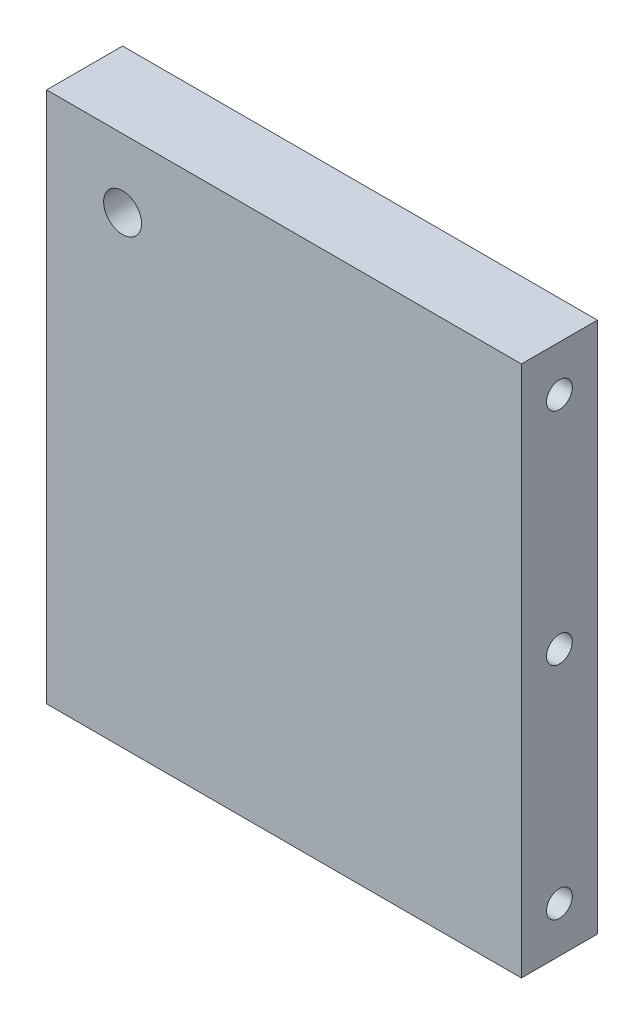
from build123d import *

# Parameters (mm, degrees)
SKETCH1_W              = 125
SKETCH1_H              = 140
BOSS_EXTRUDE1_DEPTH    = 20
M10_TAPPED_HOLE1_D     = 8.5
M10_TAPPED_HOLE1_DEPTH = 35
M10_TAPPED_HOLE1_TIP   = 2.553657631
M8_TAPPED_HOLE1_D      = 6.8
M8_TAPPED_HOLE1_DEPTH  = 22.25
M8_TAPPED_HOLE1_TIP    = 2.042926105
SKETCH6_R              = 5
CUT_EXTRUDE1_DEPTH     = 96.949205312


with BuildPart() as part:
    # Sketch1 → Boss-Extrude1 (new body)
    with BuildSketch(Plane.XY):
        Rectangle(SKETCH1_W, SKETCH1_H)
    extrude(amount=BOSS_EXTRUDE1_DEPTH)

    # M10 Tapped Hole1
    with Locations(Plane.ZY.offset(62.5)):
        with Locations((10, 40), (10, 0), (10, -40)):
            Hole(M10_TAPPED_HOLE1_D / 2, depth=M10_TAPPED_HOLE1_DEPTH)
            with Locations((0, 0, -(M10_TAPPED_HOLE1_DEPTH + M10_TAPPED_HOLE1_TIP / 2))):  # 118° drill point
                Cone(0, M10_TAPPED_HOLE1_D / 2, M10_TAPPED_HOLE1_TIP, mode=Mode.SUBTRACT)

    # M8 Tapped Hole1
    with Locations(Plane(origin=(62.5, 0, 0), x_dir=(0, 0, -1), z_dir=(1, 0, 0))):
        with Locations((-10, 58), (-10, 0), (-10, -58)):
            Hole(M8_TAPPED_HOLE1_D / 2, depth=M8_TAPPED_HOLE1_DEPTH)
            with Locations((0, 0, -(M8_TAPPED_HOLE1_DEPTH + M8_TAPPED_HOLE1_TIP / 2))):  # 118° drill point
                Cone(0, M8_TAPPED_HOLE1_D / 2, M8_TAPPED_HOLE1_TIP, mode=Mode.SUBTRACT)

    # Sketch6 → Cut-Extrude1 (cut, through all)
    with BuildSketch(Plane.XY.offset(20)):
        with Locations((-42.5, 52)):
            Circle(SKETCH6_R)
    extrude(amount=-CUT_EXTRUDE1_DEPTH, mode=Mode.SUBTRACT)


solid = part.part
